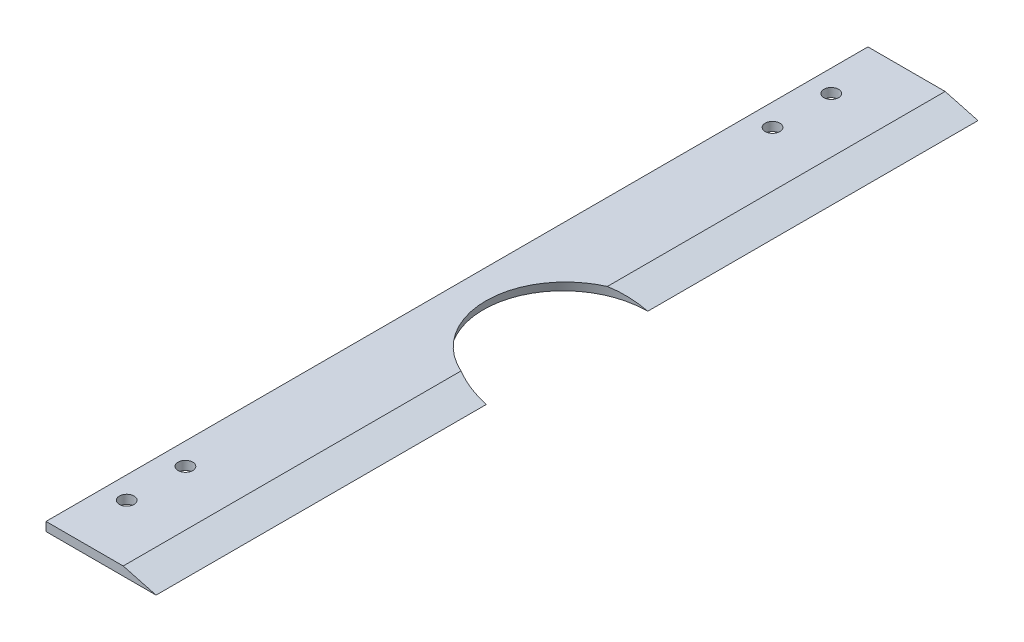
SolidWorks part; units mm, degrees
ref_plane "前视基准面" through (0, 0, 0) normal (0, 0, 1) x (1, 0, 0)
ref_plane "上视基准面" through (0, 0, 0) normal (0, 1, 0) x (1, 0, 0)
ref_plane "右视基准面" through (0, 0, 0) normal (1, 0, 0) x (0, 0, -1)
sketch "草图1" plane through (0, 0, 0) normal (0, 0, 1) x (1, 0, 0)
  line L0 (0, 0) -> (0, -3)
  line L1 (0, -3) -> (37.5, -3)
  line L2 (37.5, -3) -> (26.3038, 0)
  line L3 (26.3038, 0) -> (0, 0)
  dimension "D1" = 37.5
  dimension "D2" = 3
  dimension "D3" = 15
extrude "凸台-拉伸1" add sketch "草图1" along normal blind 280
sketch "草图2" plane through (0, 0, 0) normal (0, 1, 0) x (1, 0, 0)
  line L0 (26.3038, 0) -> (0, 0) construction
  line L1 (26.3038, -280) -> (0, -280) construction
  circle A0 centre (7.5, -260) radius 2.5
  circle A1 centre (7.5, -240) radius 2.5
  circle A2 centre (7.5, -20) radius 2.5
  circle A3 centre (7.5, -40) radius 2.5
  dimension "D1" = 20
  dimension "D2" = 20
  dimension "D3" = 20
  dimension "D4" = 20
extrude "切除-拉伸1" cut sketch "草图2" against normal blind 280
sketch "草图3" plane through (1.762, 6.576, 0) normal (0.2588, 0.9659, 0) x (0.9659, -0.2588, 0)
  line L1 (36.9987, -280) -> (36.9987, 0) construction
  line L2 (0, -280) -> (0, 0) construction
  circle A1 centre (36.9987, -140) radius 27.5
  dimension "D1" = 36.9987
  dimension "D2" = 55
extrude "切除-拉伸5" cut sketch "草图3" against normal through all
